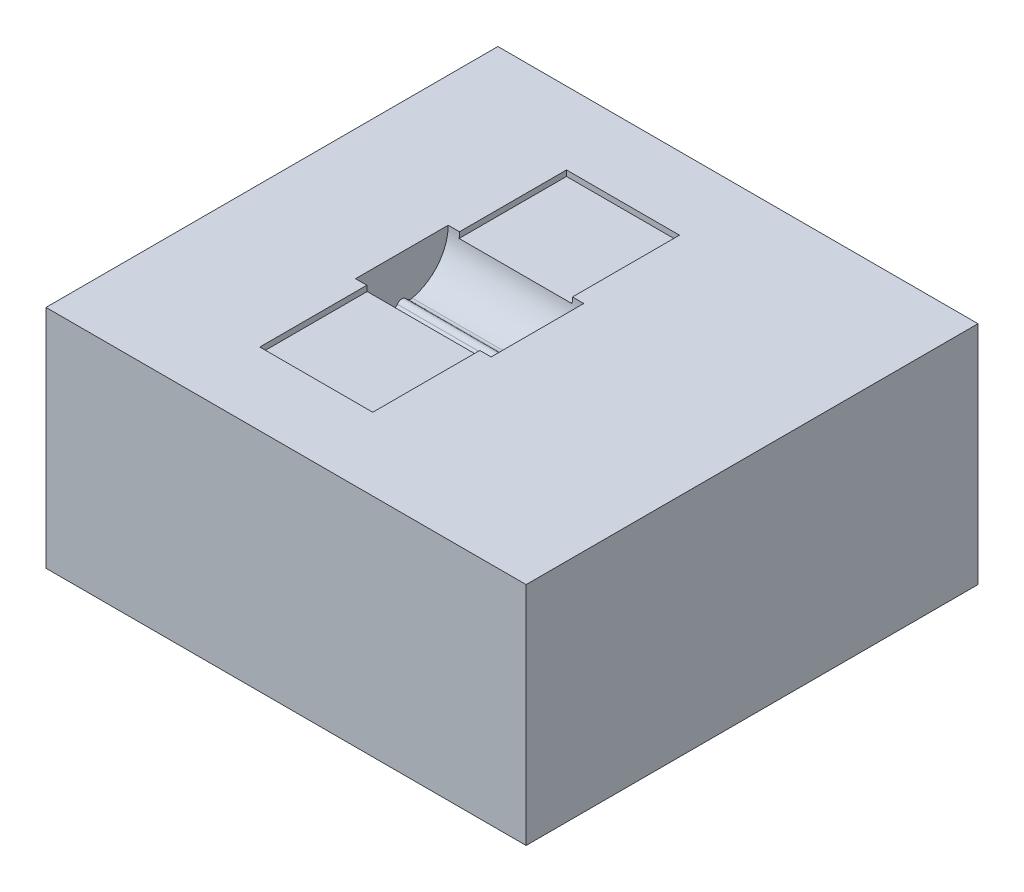
SolidWorks part; units mm, degrees
ref_plane "Front Plane" through (0, 0, 0) normal (0, 0, 1) x (1, 0, 0)
ref_plane "Top Plane" through (0, 0, 0) normal (0, 1, 0) x (1, 0, 0)
ref_plane "Right Plane" through (0, 0, 0) normal (1, 0, 0) x (0, 0, -1)
sketch "Sketch1" plane through (0, 0, 0) normal (0, 1, 0) x (1, 0, 0)
  line L1 (-42.5, -40) -> (42.5, -40)
  line L2 (-42.5, -40) -> (-42.5, 40)
  line L3 (-42.5, 40) -> (42.5, 40)
  line L4 (42.5, -40) -> (42.5, 40)
  line L5 (-42.5, -40) -> (42.5, 40) construction
  line L6 (-42.5, 40) -> (42.5, -40) construction
  point P0 (0, 0)
  dimension "D1" = 85
  dimension "D2" = 80
extrude "Boss-Extrude1" add sketch "Sketch1" along normal blind 40
hole_wizard "M8 Tapped Hole1" positions "Sketch3" profile "Sketch4" tap size "M8" standard "GB"
sketch "Sketch3" plane through (0, 0, 0) normal (0, -1, 0) x (-1, 0, 0)
  line L3 (-42.5, -40) -> (-42.5, 40) construction
  point P0 (7.5, 28)
  point P2 (-22.5, 0)
  point P4 (7.5, -28)
  point P6 (32.5, 0)
  dimension "D1" = 22.5
  dimension "D2" = 32.5
  dimension "D3" = 50
  dimension "D4" = 50
  dimension "D5" = 28
  dimension "D6" = 28
sketch "Sketch4" plane through (-7.5, 0, -28) normal (1, 0, 0) x (0, 0, -1)
  line L0 (0, 0) -> (0, 24.2929)
  line L1 (0, 24.2929) -> (3.4, 22.25)
  line L2 (3.4, 22.25) -> (3.4, 0.625)
  line L3 (3.4, 0.625) -> (4.025, 0)
  line L5 (4.025, 0) -> (0, 0)
  line L6 (-3.4, 0.625) -> (-4.025, 0) construction
  line L10 (0, 24.2929) -> (-3.4, 22.25) construction
  line L11 (0, -6.35) -> (0, 107.95) construction
  dimension "螺纹孔钻头直径" = 6.8
  dimension "螺纹孔钻头深度" = 22.25
  dimension "近端锥形沉头孔直径" = 8.05
  dimension "近端锥形沉头孔角度" = 90
  dimension "导头角度" = 118
cosmetic thread "Hole Thread Line 1"
cosmetic thread "Hole Thread Line 2"
cosmetic thread "Hole Thread Line 3"
cosmetic thread "Hole Thread Line 4"
sketch "Sketch5" plane through (0, 40, 0) normal (0, 1, 0) x (1, 0, 0)
  line L0 (42.5, -40) -> (42.5, 40) construction
  line L1 (-17.5, 27.15) -> (2.5, 27.15)
  line L2 (-17.5, 27.15) -> (-17.5, -27.15)
  line L3 (-17.5, -27.15) -> (2.5, -27.15)
  line L4 (2.5, 27.15) -> (2.5, -27.15)
  line L5 (-17.5, 27.15) -> (2.5, -27.15) construction
  line L6 (-17.5, -27.15) -> (2.5, 27.15) construction
  point P0 (-7.5, 0)
  dimension "D1" = 54.3
  dimension "D2" = 20
  dimension "D3" = 50
extrude "Cut-Extrude1" cut sketch "Sketch5" against normal blind 1
ref_plane "Plane1" through (-7.5, 0, 0) normal (-1, 0, 0) x (0, 0, 1)
sketch "Sketch6" plane through (-7.5, 0, 0) normal (-1, 0, 0) x (0, 0, 1)
  line L0 (0, -1000) -> (0, 49000) construction
  line L1 (-40, 40) -> (40, 40) construction
  line L3 (-8.2, 40) -> (8.2, 40)
  arc A2 (-8.2, 40) -> (-1.8366, 32.0083) centre (0, 40) ccw
  arc A3 (0.8063, 32.3915) -> (-0.8063, 32.3915) centre (0, 31.8) ccw
  arc A4 (1.8366, 32.0083) -> (8.2, 40) centre (0, 40) ccw
  arc A5 (-0.8063, 32.3915) -> (-1.8366, 32.0083) centre (-1.6127, 32.9829) cw
  arc A6 (0.8063, 32.3915) -> (1.8366, 32.0083) centre (1.6127, 32.9829) ccw
  point P15 (0.9981, 31.861)
  dimension "D1" = 16.4
  dimension "D3" = 1
  dimension "D2" = 2
extrude "Cut-Extrude2" cut sketch "Sketch6" against normal mid plane 24
